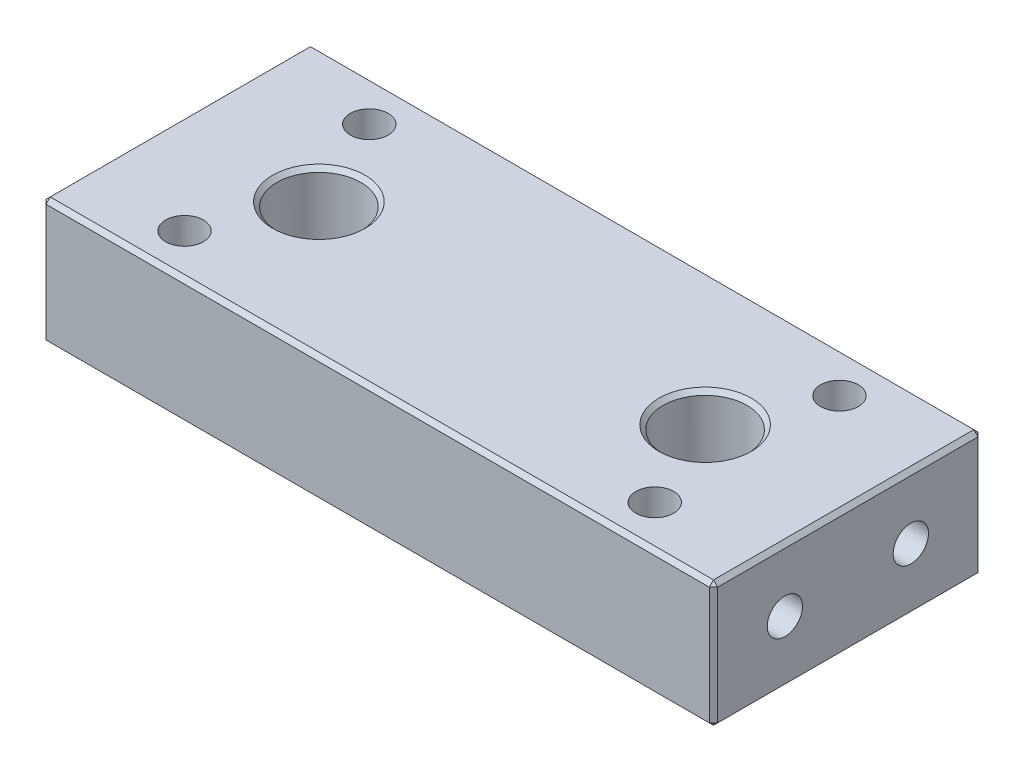
from build123d import *

# Parameters (mm, degrees)
SKETCH1_W                                            = 80
SKETCH1_H                                            = 15
EXTRUDE_THIN1_DEPTH                                  = 16
HOLE_SIZE_BY_SOCKET_HEAD_CAP_SCREW_TYPE1_D           = 4.5
HOLE_SIZE_BY_SOCKET_HEAD_CAP_SCREW_TYPE1_CBORE_D     = 8
HOLE_SIZE_BY_SOCKET_HEAD_CAP_SCREW_TYPE1_CBORE_DEPTH = 4.6
SKETCH4_R                                            = 5
CUT_EXTRUDE1_DEPTH                                   = 83.95179323
M5_TAPPED_HOLE2_D                                    = 4.2
M5_TAPPED_HOLE2_DEPTH                                = 10
M5_TAPPED_HOLE2_TIP                                  = 1.2618073
M5_TAPPED_HOLE1_D                                    = 4.2
M5_TAPPED_HOLE1_DEPTH                                = 10
M5_TAPPED_HOLE1_TIP                                  = 1.2618073
CHAMFER1_SIZE                                        = 0.5


with BuildPart() as part:
    # Sketch1 → Extrude-Thin1 (new, symmetric)
    with BuildSketch(Plane.XY):
        with Locations((40, -7.5)):
            Rectangle(SKETCH1_W, SKETCH1_H)
    extrude(amount=EXTRUDE_THIN1_DEPTH, both=True)

    # Hole size by socket head cap screw type1 (through all)
    with Locations(Plane(origin=(0, -15, 0), x_dir=(-1, 0, 0), z_dir=(0, -1, 0))):
        with Locations((-68, -11), (-68, 11), (-12, -11), (-12, 11)):
            CounterBoreHole(HOLE_SIZE_BY_SOCKET_HEAD_CAP_SCREW_TYPE1_D / 2, HOLE_SIZE_BY_SOCKET_HEAD_CAP_SCREW_TYPE1_CBORE_D / 2, HOLE_SIZE_BY_SOCKET_HEAD_CAP_SCREW_TYPE1_CBORE_DEPTH)

    # Sketch4 → Cut-Extrude1 (cut, through all)
    with BuildSketch(Plane.XZ.offset(15)):
        with Locations(Location((17, 0, 0), (0, 0, 270))):
            Circle(SKETCH4_R)
        with Locations(Location((63, 0, 0), (0, 0, 270))):
            Circle(SKETCH4_R)
    extrude(amount=-CUT_EXTRUDE1_DEPTH, mode=Mode.SUBTRACT)

    # M5 Tapped Hole2
    with Locations(Plane(origin=(80, 0, 0), x_dir=(0, 0, -1), z_dir=(1, 0, 0))):
        with Locations((-7.5, -7.5), (7.5, -7.5)):
            Hole(M5_TAPPED_HOLE2_D / 2, depth=M5_TAPPED_HOLE2_DEPTH)
            with Locations((0, 0, -(M5_TAPPED_HOLE2_DEPTH + M5_TAPPED_HOLE2_TIP / 2))):  # 118° drill point
                Cone(0, M5_TAPPED_HOLE2_D / 2, M5_TAPPED_HOLE2_TIP, mode=Mode.SUBTRACT)

    # M5 Tapped Hole1
    with Locations(Plane(origin=(0, -24.315194206, 11.709083439), x_dir=(0, 0, 1), z_dir=(-1, 0, 0))):
        with Locations((-19.209083439, 16.815194206), (-4.209083439, 16.815194206)):
            Hole(M5_TAPPED_HOLE1_D / 2, depth=M5_TAPPED_HOLE1_DEPTH)
            with Locations((0, 0, -(M5_TAPPED_HOLE1_DEPTH + M5_TAPPED_HOLE1_TIP / 2))):  # 118° drill point
                Cone(0, M5_TAPPED_HOLE1_D / 2, M5_TAPPED_HOLE1_TIP, mode=Mode.SUBTRACT)

    # Chamfer1
    chamfer1_edges = [part.edges().sort_by_distance(p)[0] for p in [
        (40, 0, 16),
        (0, -7.5, 16),
        (0, -7.5, -16),
        (40, -15, 16),
        (40, 0, -16),
        (17, 0, 5),
        (17, -15, 5),
        (80, -7.5, -16),
        (63, 0, 5),
        (63, -15, 5),
        (40, -15, -16),
        (0, -15, 0),
        (0, 0, 0),
        (80, 0, 0),
        (80, -15, 0),
        (80, -7.5, 16),
    ]]
    chamfer(chamfer1_edges, length=CHAMFER1_SIZE)


solid = part.part
